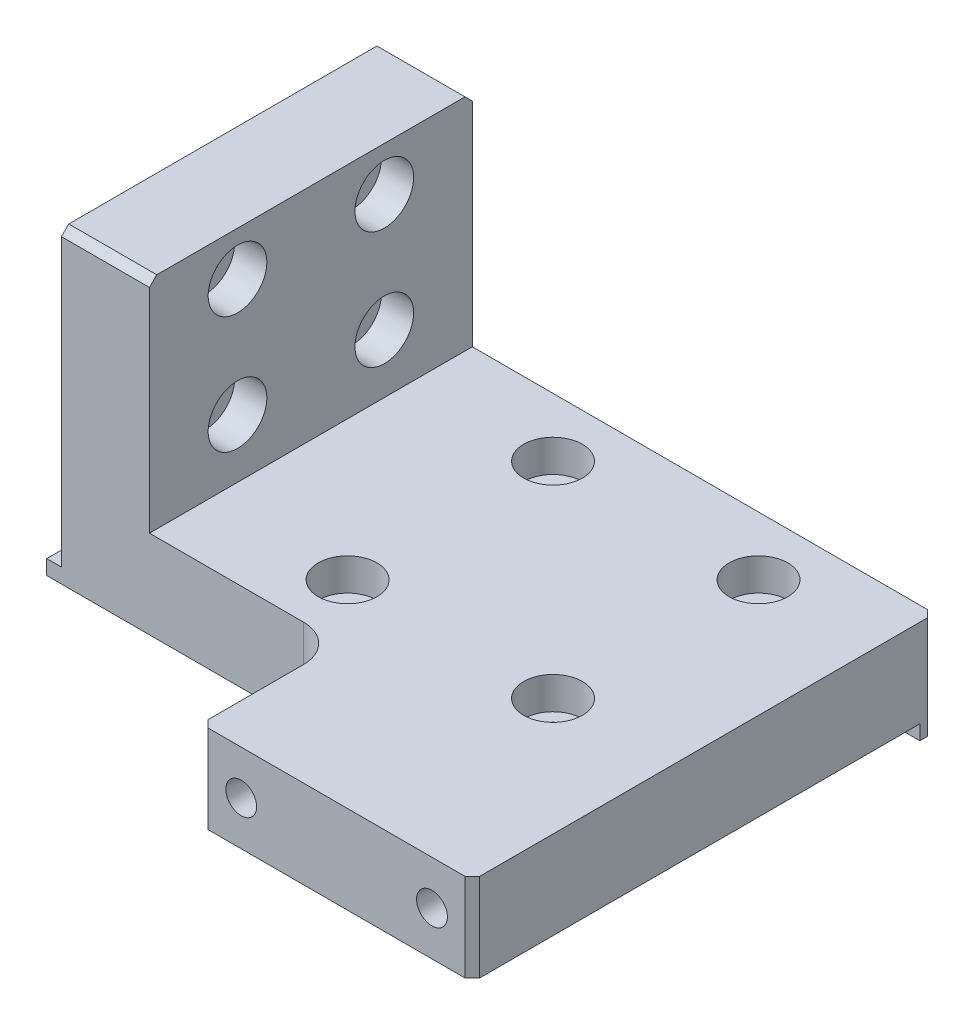
SolidWorks part; units mm, degrees
material "SS41"
ref_plane "Front Plane" through (0, 0, 0) normal (0, 0, 1) x (1, 0, 0)
ref_plane "Top Plane" through (0, 0, 0) normal (0, 1, 0) x (1, 0, 0)
ref_plane "Right Plane" through (0, 0, 0) normal (1, 0, 0) x (0, 0, -1)
sketch "Sketch1" plane through (0, 0, 0) normal (0, 0, 1) x (1, 0, 0)
  line L1 (-37.5, 6) -> (37.5, 6)
  line L2 (-37.5, 6) -> (-37.5, -6)
  line L3 (-37.5, -6) -> (37.5, -6)
  line L4 (37.5, 6) -> (37.5, -6)
  line L5 (-37.5, 6) -> (37.5, -6) construction
  line L6 (-37.5, -6) -> (37.5, 6) construction
  point P0 (0, 0)
  dimension "D1" = 75
  dimension "D2" = 12
extrude "Boss-Extrude1" add sketch "Sketch1" along normal blind 73
sketch "Sketch2" plane through (0, -6, 0) normal (0, -1, 0) x (1, 0, 0)
  line L0 (-37.5, 73) -> (-37.5, 0) construction
  line L1 (37.5, 0) -> (-37.5, 0)
  line L2 (37.5, 0) -> (37.5, 2)
  line L3 (37.5, 2) -> (-37.5, 2)
  line L4 (-37.5, 0) -> (-37.5, 2)
  dimension "D1" = 2
extrude "Boss-Extrude2" add sketch "Sketch2" along normal blind 2
sketch "Sketch3" plane through (0, 6, 0) normal (0, 1, 0) x (1, 0, 0)
  line L0 (-37.5, -73) -> (-37.5, 0) construction
  line L1 (37.5, -73) -> (-37.5, -73)
  line L2 (37.5, -73) -> (37.5, -63)
  line L3 (37.5, -63) -> (-37.5, -63)
  line L4 (-37.5, -73) -> (-37.5, -63)
  dimension "D1" = 10
extrude "Boss-Extrude3" add sketch "Sketch3" along normal blind 15
sketch "Sketch4" plane through (0, 6, 0) normal (0, 1, 0) x (1, 0, 0)
  line L0 (37.5, 0) -> (-37.5, 0) construction
  line L1 (-37.5, -63) -> (-25.5, -63)
  line L2 (-37.5, -63) -> (-37.5, 0)
  line L3 (-37.5, 0) -> (-25.5, 0)
  line L4 (-25.5, -63) -> (-25.5, 0)
  dimension "D1" = 12
extrude "Boss-Extrude4" add sketch "Sketch4" along normal blind 30
sketch "Sketch5" plane through (-37.5, 0, 0) normal (-1, 0, 0) x (0, 0, 1)
  line L0 (0, 36) -> (0, -8) construction
  line L1 (0, -6) -> (63, -6)
  line L2 (0, -6) -> (0, -4)
  line L3 (0, -4) -> (63, -4)
  line L4 (63, -6) -> (63, -4)
  line L5 (73, -6) -> (2, -6) construction
  line L6 (63, 36) -> (63, 21) construction
  dimension "D1" = 2
extrude "Boss-Extrude5" add sketch "Sketch5" along normal blind 2
sketch "Sketch7" plane through (0, 0, 73) normal (0, 0, 1) x (1, 0, 0)
  line L1 (-39.5, -6) -> (0.5, -6)
  line L2 (-39.5, -6) -> (-39.5, 36)
  line L3 (-39.5, 36) -> (0.5, 36)
  line L4 (0.5, -6) -> (0.5, 36)
  line L5 (-37.5, 36) -> (-25.5, 36) construction
  dimension "D1" = 40
extrude "Cut-Extrude2" cut sketch "Sketch7" against normal blind 29
hole_wizard "M5 Tapped Hole1" positions "Sketch9" profile "Sketch8" tap size "M5" standard "Iso"
sketch "Sketch9" plane through (0, 0, 73) normal (0, 0, 1) x (1, 0, 0)
  line L1 (19, 21) -> (19, -8) construction
  line L2 (0.5, 21) -> (37.5, 21) construction
  line L3 (37.5, -8) -> (-37.5, -8) construction
  point P0 (19, 10)
  dimension "D1" = 11
sketch "Sketch8" plane through (19, 10, 73) normal (1, 0, 0) x (0, -1, 0)
  line L0 (0, 0) -> (0, 13.6618)
  line L1 (0, 13.6618) -> (2.1, 12.4)
  line L2 (2.1, 12.4) -> (2.1, 0)
  line L5 (2.1, 0) -> (0, 0)
  line L10 (0, 13.6618) -> (-2.1, 12.4) construction
  line L11 (0, -6.35) -> (0, 107.95) construction
  dimension "螺纹孔钻头直径" = 4.2
  dimension "螺纹孔钻头深度" = 12.4
  dimension "导头角度" = 118
cosmetic thread "Hole thread1" parameters "D1"=10, "D2"=5
hole_wizard "CBORE for M4 Hex Socket Head Cap Screw1" positions "Sketch11" profile "Sketch10" counterbore size "M4" standard "Iso" end condition through all
sketch "Sketch11" plane through (-25.5, 0, 0) normal (1, 0, 0) x (0, 0, -1)
  line L0 (-22, 36) -> (-22, 8.0233) construction
  line L1 (-44, 36) -> (0, 36) construction
  point P0 (-32, 30)
  point P2 (-32, 14)
  point P13 (-12, 14)
  point P14 (-12, 30)
  dimension "D1" = 6
  dimension "D2" = 10
  dimension "D3" = 16
sketch "Sketch10" plane through (-25.5, 30, 32) normal (0, 1, 0) x (0, 0, -1)
  line L0 (0, 0) -> (0, 14)
  line L1 (0, 14) -> (2.25, 14)
  line L3 (2.25, 14) -> (2.25, 4.4)
  line L4 (2.25, 4.4) -> (4, 4.4)
  line L5 (4, 4.4) -> (4, 0)
  line L7 (4, 0) -> (0, 0)
  line L11 (0, -6.35) -> (0, 107.95) construction
  dimension "通孔孔直径" = 4.5
  dimension "通孔孔深度" = 14
  dimension "柱形沉头孔直径" = 8
  dimension "柱形沉头孔深度" = 4.4
sketch "Sketch12" plane through (0, 21, 0) normal (0, 1, 0) x (1, 0, 0)
  line L0 (0.5, -73) -> (0.5, -63) construction
  line L1 (37.5, -73) -> (0.5, -73)
  line L2 (37.5, -73) -> (37.5, -63)
  line L3 (37.5, -63) -> (0.5, -63)
  line L4 (0.5, -73) -> (0.5, -63)
  line L5 (37.5, -63) -> (0.5, -63) construction
  line L6 (37.5, -63) -> (0.5, -63) construction
extrude "Cut-Extrude3" cut sketch "Sketch12" against normal through all
hole_wizard "M5 Tapped Hole2" positions "Sketch14" profile "Sketch13" tap size "M5" standard "Iso"
sketch "Sketch14" plane through (0, 0, 63) normal (0, 0, 1) x (1, 0, 0)
  line L0 (19, 6) -> (19, -6) construction
  line L1 (37.5, 6) -> (0.5, 6) construction
  line L2 (37.5, -6) -> (0.5, -6) construction
  point P0 (32, 0)
  point P2 (6, 0)
  dimension "D1" = 6
  dimension "D2" = 26
sketch "Sketch13" plane through (32, 0, 63) normal (1, 0, 0) x (0, -1, 0)
  line L0 (0, 0) -> (0, 13.6618)
  line L1 (0, 13.6618) -> (2.1, 12.4)
  line L2 (2.1, 12.4) -> (2.1, 0)
  line L5 (2.1, 0) -> (0, 0)
  line L10 (0, 13.6618) -> (-2.1, 12.4) construction
  line L11 (0, -6.35) -> (0, 107.95) construction
  dimension "螺纹孔钻头直径" = 4.2
  dimension "螺纹孔钻头深度" = 12.4
  dimension "导头角度" = 118
cosmetic thread "Hole thread2" parameters "D1"=10, "D2"=5
cosmetic thread "Hole thread3" parameters "D1"=10, "D2"=5
fillet "Fillet1" radius 5 1 edges at (0.5, 0, 44)
hole_wizard "CBORE for M4 Hex Socket Head Cap Screw2" positions "Sketch16" profile "Sketch15" counterbore size "M4" standard "Iso" end condition through all
sketch "Sketch16" plane through (0, 6, 0) normal (0, 1, 0) x (1, 0, 0)
  line L0 (-25.5, -22) -> (37.5, -22) construction
  line L1 (-25.5, -44) -> (-25.5, 0) construction
  line L2 (37.5, -63) -> (37.5, 0) construction
  point P0 (-6.5, -8)
  point P3 (21.5, -8)
  point P6 (-6.5, -36)
  point P9 (21.5, -36)
  dimension "D1" = 28
  dimension "D2" = 28
  dimension "D3" = 16
sketch "Sketch15" plane through (-6.5, 6, 8) normal (1, 0, 0) x (0, 0, 1)
  line L0 (0, 0) -> (0, 14)
  line L1 (0, 14) -> (2.25, 14)
  line L3 (2.25, 14) -> (2.25, 4.4)
  line L4 (2.25, 4.4) -> (4, 4.4)
  line L5 (4, 4.4) -> (4, 0)
  line L7 (4, 0) -> (0, 0)
  line L11 (0, -6.35) -> (0, 107.95) construction
  dimension "通孔孔直径" = 4.5
  dimension "通孔孔深度" = 14
  dimension "柱形沉头孔直径" = 8
  dimension "柱形沉头孔深度" = 4.4
chamfer "Chamfer1" distance 1 angle 45 5 edges at (0.5, 0, 63) (37.5, -1, 0) (-31.5, 36, 0) (-31.5, 36, 44)
